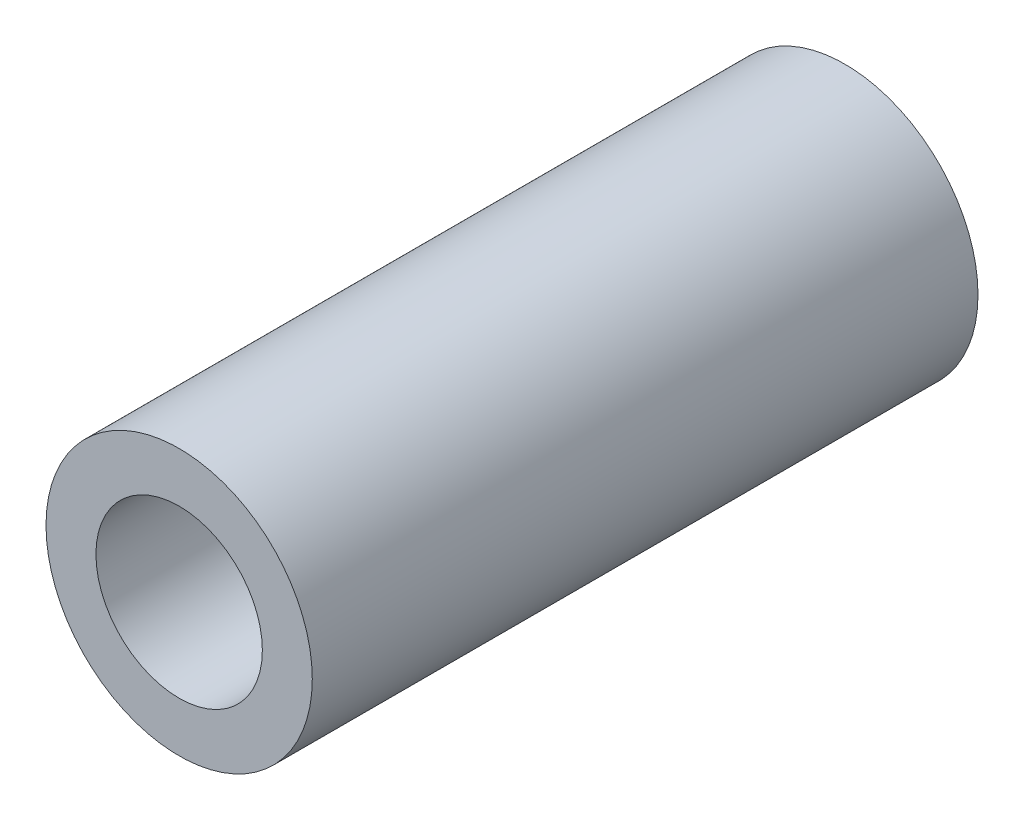
from build123d import *

# Parameters (mm, degrees)
SKETCH1_R           = 8
BOSS_EXTRUDE1_DEPTH = 40
SKETCH2_R           = 5
CUT_EXTRUDE1_DEPTH  = 33


with BuildPart() as part:
    # Sketch1 → Boss-Extrude1 (new body)
    with BuildSketch(Plane.XY):
        Circle(SKETCH1_R)
    extrude(amount=BOSS_EXTRUDE1_DEPTH)

    # Sketch2 → Cut-Extrude1 (cut)
    with BuildSketch(Plane.XY.offset(40)):
        Circle(SKETCH2_R)
    extrude(amount=-CUT_EXTRUDE1_DEPTH, mode=Mode.SUBTRACT)


solid = part.part
